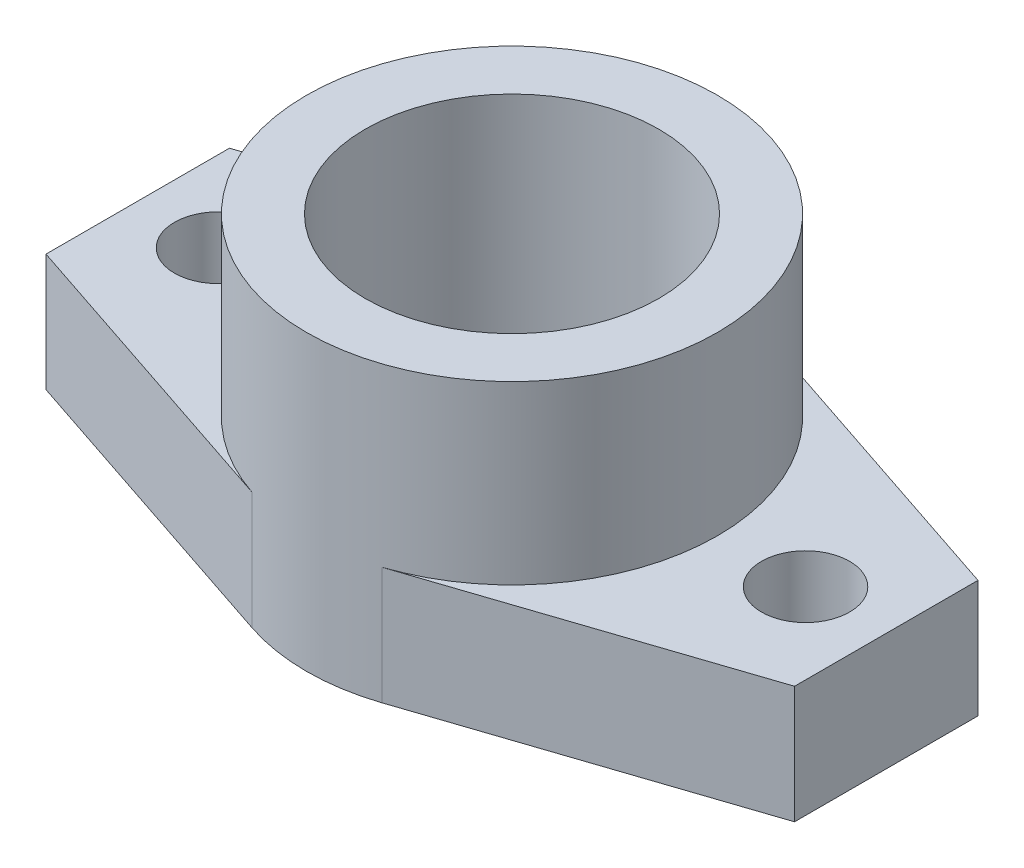
from build123d import *

# Parameters (mm, degrees)
SKETCH_1_R          = 28
EXTRUDE_1_DEPTH     = 40
EXTRUDE_2_DEPTH     = 16
SKETCH_3_R          = 20
CUT_EXTRUDE_1_DEPTH = 71.604532432
SKETCH_4_R          = 6
CUT_EXTRUDE_2_DEPTH = 63.93647591


with BuildPart() as part:
    # 草图1 → 凸台-拉伸1 (new body)
    with BuildSketch(Plane(origin=(0, 0, 0), x_dir=(1, 0, 0), z_dir=(0, 1, 0))):
        with Locations(Location((0, 0, 0), (0, 0, 270))):
            Circle(SKETCH_1_R)
    extrude(amount=EXTRUDE_1_DEPTH)

    # 草图2 → 凸台-拉伸2 (add)
    with BuildSketch(Plane.XZ):
        Polygon((-51, -12.5), (-51, 12.5), (-8.862653898, 26.560372096), (-8.862653898, -26.560372096), align=None)
    extrude_2 = extrude(amount=-EXTRUDE_2_DEPTH)

    # 镜向1: 凸台-拉伸2 across plane
    add(extrude_2.mirror(Plane(origin=(0, 0, 0), x_dir=(0, 0, 1), z_dir=(1, 0, 0))))

    # 草图3 → 切除-拉伸1 (cut, through all)
    with BuildSketch(Plane(origin=(0, 40, 0), x_dir=(1, 0, 0), z_dir=(0, 1, 0))):
        with Locations(Location((0, 0, 0), (0, 0, 270))):
            Circle(SKETCH_3_R)
    extrude(amount=-CUT_EXTRUDE_1_DEPTH, mode=Mode.SUBTRACT)

    # 草图4 → 切除-拉伸2 (cut, through all)
    with BuildSketch(Plane(origin=(0, 16, 0), x_dir=(1, 0, 0), z_dir=(0, 1, 0))):
        with Locations(Location((-40, 0, 0), (0, 0, 270))):
            Circle(SKETCH_4_R)
        with Locations(Location((40, 0, 0), (0, 0, 270))):
            Circle(SKETCH_4_R)
    extrude(amount=-CUT_EXTRUDE_2_DEPTH, mode=Mode.SUBTRACT)


solid = part.part
